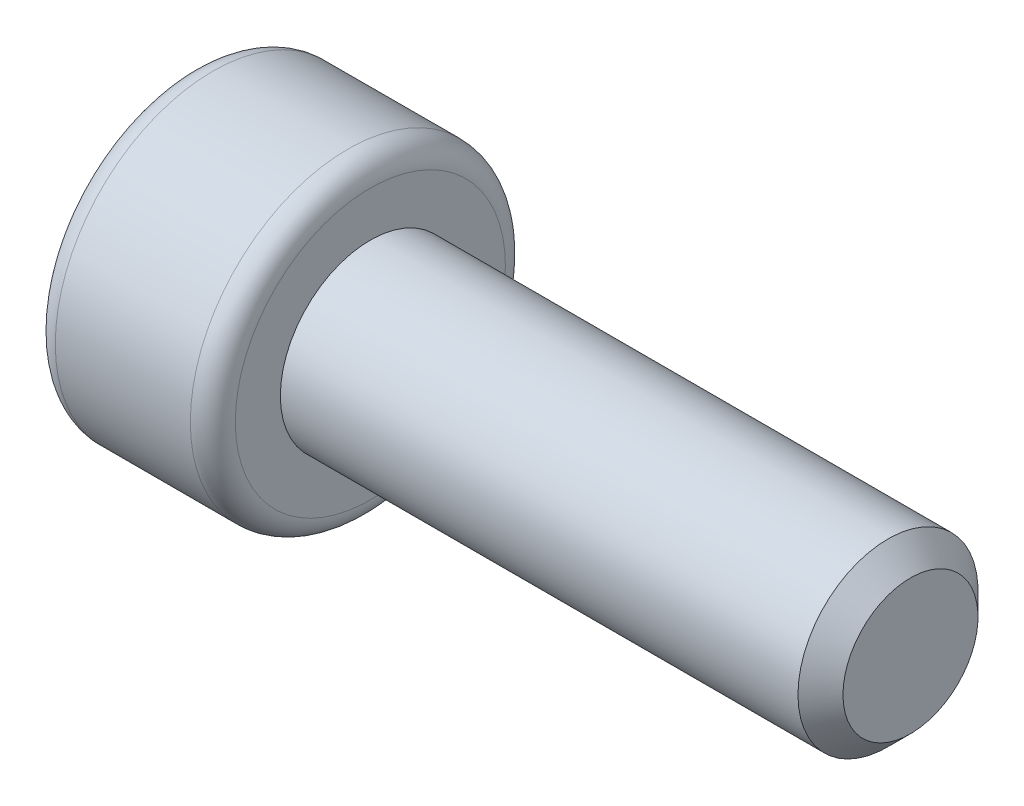
from build123d import *

# Parameters (mm, degrees)
CUT_EXTRUDE1_DEPTH = 2
FILLET1_R          = 0.5
CHAMFER1_SIZE      = 0.1
CHAMFER1_SIZE2     = 0.567128182
CHAMFER2_SIZE      = 0.5


with BuildPart() as part:
    # Sketch1 → Revolve1 (revolve)
    with BuildSketch(Plane.XY, mode=Mode.PRIVATE) as revolve1_sk:
        Polygon((0, 0), (0, 3.5), (4, 3.5), (4, 2), (16, 2), (16, 0), align=None)
    revolve(revolve1_sk.sketch.rotate(Axis((-4.709244637, 0, 0), (1, 0, 0)), 90), axis=Axis((-4.709244637, 0, 0), (1, 0, 0)))

    # Sketch4 → Cut-Extrude1 (cut)
    with BuildSketch(Plane.ZY):
        Polygon((-1.732050808, 0), (-0.866025404, -1.5), (0.866025404, -1.5), (1.732050808, 0), (0.866025404, 1.5), (-0.866025404, 1.5), align=None)
    extrude(amount=-CUT_EXTRUDE1_DEPTH, mode=Mode.SUBTRACT)

    # Fillet1
    fillet1_edges = [part.edges().sort_by_distance(p)[0] for p in [
        (4, 0, -3.5),
        (0, 0, -3.5),
    ]]
    fillet(fillet1_edges, radius=FILLET1_R)

    # Chamfer1
    chamfer1_edges = [part.edges().sort_by_distance(p)[0] for p in [
        (0, 0.75, -1.299038106),
        (0, -0.75, -1.299038106),
        (0, -1.5, 0),
        (0, -0.75, 1.299038106),
        (0, 0.75, 1.299038106),
        (0, 1.5, 0),
    ]]
    chamfer1_side = [part.faces().sort_by_distance(p)[0] for p in [
        (0, 0, -2.915147186),
    ]]
    chamfer(chamfer1_edges, length=CHAMFER1_SIZE, length2=CHAMFER1_SIZE2, reference=chamfer1_side[0])

    # Chamfer2
    chamfer2_edges = [part.edges().sort_by_distance(p)[0] for p in [
        (16, 0, -2),
    ]]
    chamfer(chamfer2_edges, length=CHAMFER2_SIZE)


solid = part.part
